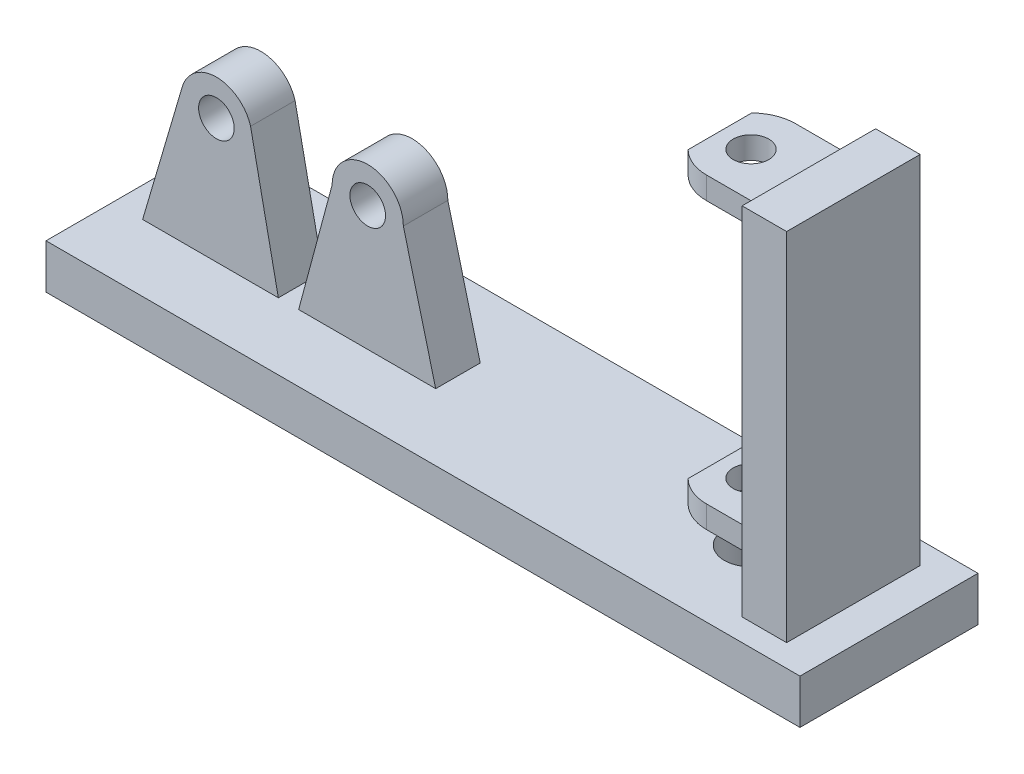
SolidWorks part; units mm, degrees
ref_plane "Front Plane" through (0, 0, 0) normal (0, 0, 1) x (1, 0, 0)
ref_plane "Top Plane" through (0, 0, 0) normal (0, 1, 0) x (1, 0, 0)
ref_plane "Right Plane" through (0, 0, 0) normal (1, 0, 0) x (0, 0, -1)
sketch "Sketch1" plane through (0, 0, 0) normal (0, 0, 1) x (1, 0, 0)
  line L0 (-7.6745, 2.2586) -> (-16.5796, -28)
  line L1 (-16.5796, -28) -> (-22.3531, -38)
  line L2 (-22.3531, -38) -> (137.6469, -38)
  line L3 (137.6469, -38) -> (131.8734, -28)
  line L4 (26, 0) -> (18.4767, -28)
  line L5 (0, 0) -> (0, -48.1889) construction
  line L6 (7.6745, 2.2586) -> (13.9167, -28)
  line L7 (49.355, -28.3173) -> (42, 0)
  line L8 (13.9167, -28) -> (18.4767, -28)
  line L9 (131.8734, -28) -> (49.355, -28.3173)
  line L13 (0, 0) -> (259.086, 0) construction
  circle A0 centre (0, 0) radius 4
  arc A1 (7.6745, 2.2586) -> (-7.6745, 2.2586) centre (0, 0) ccw
  circle A2 centre (34, 0) radius 4
  arc A3 (42, 0) -> (26, 0) centre (34, 0) ccw
  point P3 (159, 0)
  dimension "D1" = 8
  dimension "D2" = 16
  dimension "D3" = 38
  dimension "D6" = 8
  dimension "D10" = 16
  dimension "D11" = 34
  dimension "D4" = 60
  dimension "D5" = 160
  dimension "D7" = 60
  dimension "D8" = 10
  dimension "D9" = 10
  dimension "D12" = 10
extrude "Boss-Extrude1" add sketch "Sketch1" along normal blind 10
sketch "Sketch2" plane through (0, -38, 0) normal (0, -1, 0) x (-1, 0, 0)
  line L0 (22.3531, -10) -> (-137.6469, -10) construction
  line L1 (-146.1162, 15) -> (23.2878, 15)
  line L2 (-146.1162, 15) -> (-146.1162, -25)
  line L3 (-146.1162, -25) -> (23.2878, -25)
  line L4 (23.2878, 15) -> (23.2878, -25)
  line L5 (-146.1162, 15) -> (23.2878, -25) construction
  line L6 (-146.1162, -25) -> (23.2878, 15) construction
  point P0 (-61.4142, -5)
  dimension "D1" = 40
  dimension "D2" = 5
extrude "Boss-Extrude2" add sketch "Sketch2" against normal blind 10
sketch "Sketch3" plane through (0, -28, 0) normal (0, 1, 0) x (1, 0, 0)
  line L0 (146.1162, 15) -> (146.1162, -25) construction
  line L1 (128.1162, 10) -> (138.1162, 10)
  line L2 (128.1162, 10) -> (128.1162, -20)
  line L3 (128.1162, -20) -> (138.1162, -20)
  line L4 (138.1162, 10) -> (138.1162, -20)
  line L5 (128.1162, 10) -> (138.1162, -20) construction
  line L6 (128.1162, -20) -> (138.1162, 10) construction
  line L7 (146.1162, -25) -> (-23.2878, -25) construction
  point P0 (133.1162, -5)
  dimension "D1" = 10
  dimension "D2" = 30
  dimension "D3" = 8
  dimension "D4" = 5
extrude "Boss-Extrude3" add sketch "Sketch3" along normal blind 80
sketch "Sketch4" plane through (128.1162, 0, 0) normal (-1, 0, 0) x (0, 0, 1)
  line L0 (20, 52) -> (20, -28) construction
  line L1 (-5, 49) -> (15, 49)
  line L2 (-5, 49) -> (-5, 44)
  line L3 (-5, 44) -> (15, 44)
  line L4 (15, 49) -> (15, 44)
  line L5 (-5, 49) -> (15, 44) construction
  line L6 (-5, 44) -> (15, 49) construction
  line L7 (-5, -15) -> (15, -15)
  line L8 (-5, -15) -> (-5, -20)
  line L9 (-5, -20) -> (15, -20)
  line L10 (15, -15) -> (15, -20)
  line L11 (-5, -15) -> (15, -20) construction
  line L12 (-5, -20) -> (15, -15) construction
  line L13 (-10, -28) -> (20, -28) construction
  line L14 (-10, 52) -> (20, 52) construction
  point P0 (5, 46.5)
  point P5 (5, -17.5)
  dimension "D1" = 5
  dimension "D2" = 20
  dimension "D3" = 20
  dimension "D4" = 5
  dimension "D5" = 5
  dimension "D6" = 5
  dimension "D7" = 8
  dimension "D8" = 3
extrude "Boss-Extrude4" add sketch "Sketch4" along normal blind 20
sketch "Sketch5" plane through (0, 49, 0) normal (0, 1, 0) x (1, 0, 0)
  line L0 (115.1162, -15) -> (103.1743, -18.1139)
  line L1 (103.1743, -18.1139) -> (97.1472, 5)
  line L2 (97.1472, 5) -> (115.1162, 5)
  line L3 (108.1162, -15) -> (128.1162, -15) construction
  line L4 (108.1162, -15) -> (108.1162, 5) construction
  circle A0 centre (115.1162, -5) radius 4
  arc A1 (115.1162, 5) -> (115.1162, -15) centre (115.1162, -5) ccw
  dimension "D1" = 8
  dimension "D2" = 10
  dimension "D3" = 10
  dimension "D4" = 7
extrude "Cut-Extrude1" cut sketch "Sketch5" against normal blind 70
sketch "Sketch6" plane through (0, -28, 0) normal (0, 1, 0) x (1, 0, 0)
  circle A0 centre (115.1162, -5) radius 6
  dimension "D1" = 12
extrude "Cut-Extrude2" cut sketch "Sketch6" against normal blind 30
